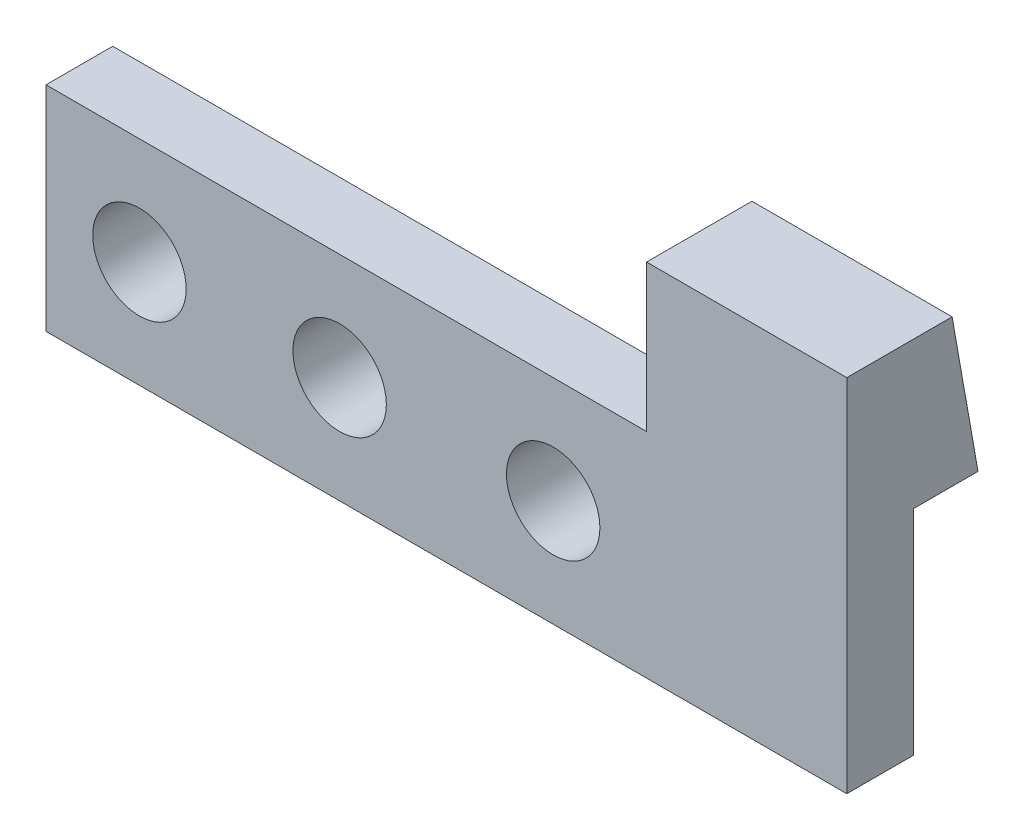
from build123d import *

# Parameters (mm, degrees)
BOSS_EXTRUDE1_DEPTH = 60
SKETCH2_W           = 45
SKETCH2_H           = 11
CUT_EXTRUDE1_DEPTH  = 60
SKETCH3_R           = 3.5
CUT_EXTRUDE2_DEPTH  = 60


with BuildPart() as part:
    # Sketch1 → Boss-Extrude1 (new body)
    with BuildSketch(Plane(origin=(0, 0, 0), x_dir=(0, 0, -1), z_dir=(1, 0, 0))):
        Polygon((0, 0), (0, 27), (7.89031, 27), (9.829906784, 16), (5, 16), (5, 0), align=None)
    extrude(amount=BOSS_EXTRUDE1_DEPTH)

    # Sketch2 → Cut-Extrude1 (cut)
    with BuildSketch(Plane.XY):
        with Locations((22.5, 21.5)):
            Rectangle(SKETCH2_W, SKETCH2_H)
    extrude(amount=-CUT_EXTRUDE1_DEPTH, mode=Mode.SUBTRACT)

    # Sketch3 → Cut-Extrude2 (cut)
    with BuildSketch(Plane.XY):
        with Locations((7, 8)):
            Circle(SKETCH3_R)
        with Locations((22, 8)):
            Circle(SKETCH3_R)
        with Locations((38, 8)):
            Circle(SKETCH3_R)
    extrude(amount=-CUT_EXTRUDE2_DEPTH, mode=Mode.SUBTRACT)


solid = part.part
